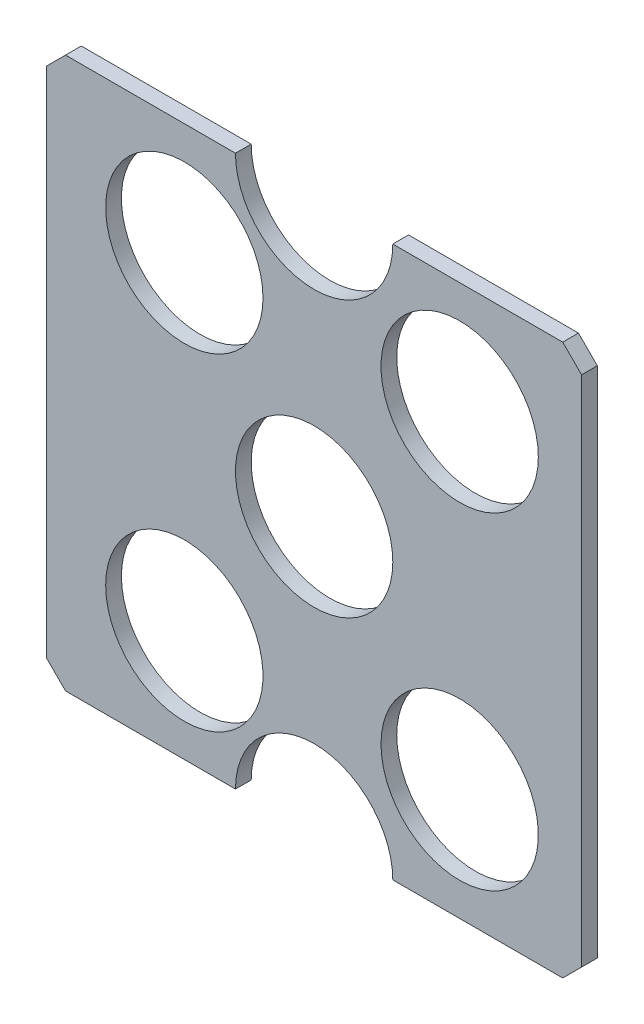
from build123d import *

# Parameters (mm, degrees)
SKETCH1_R           = 50
BOSS_EXTRUDE1_DEPTH = 10


with BuildPart() as part:
    # Sketch1 → Boss-Extrude1 (new body)
    with BuildSketch(Plane.XY):
        with BuildLine():
            Line((12, 0), (120, 0))
            ThreePointArc((120, 0), (170, 50), (220, 0))
            Line((220, 0), (328, 0))
            Line((328, 0), (340, 12))
            Line((340, 12), (340, 338))
            Line((340, 338), (328, 350))
            Line((328, 350), (220, 350))
            ThreePointArc((220, 350), (170, 300), (120, 350))
            Line((120, 350), (12, 350))
            Line((12, 350), (0, 338))
            Line((0, 338), (0, 12))
            Line((0, 12), (12, 0))
        make_face()
        with Locations((170, 175)):
            Circle(SKETCH1_R, mode=Mode.SUBTRACT)
        with Locations((87.5, 279)):
            Circle(SKETCH1_R, mode=Mode.SUBTRACT)
        with Locations((262.5, 279)):
            Circle(SKETCH1_R, mode=Mode.SUBTRACT)
        with Locations(Location((87.5, 71, 0), (0, 0, 180))):
            Circle(SKETCH1_R, mode=Mode.SUBTRACT)
        with Locations(Location((262.5, 71, 0), (0, 0, 180))):
            Circle(SKETCH1_R, mode=Mode.SUBTRACT)
    extrude(amount=BOSS_EXTRUDE1_DEPTH)


solid = part.part
